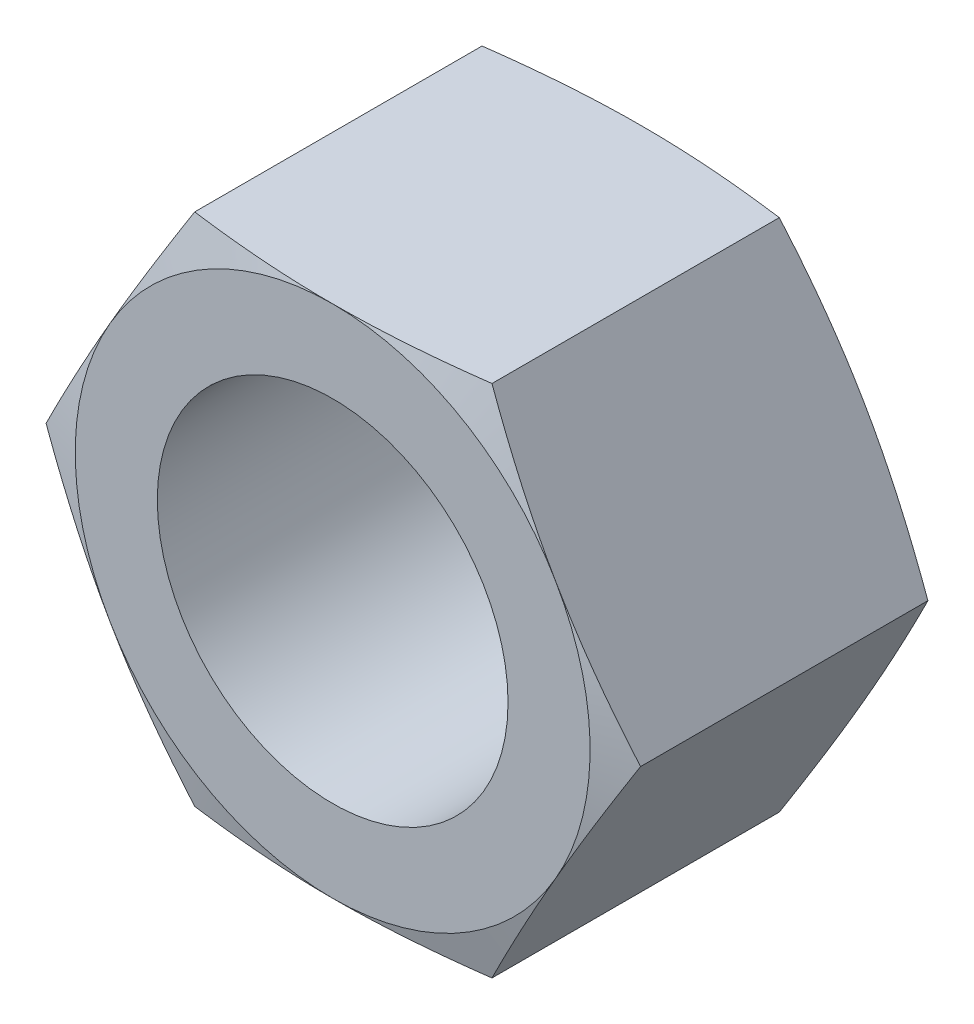
SolidWorks part; units mm, degrees
ref_plane "基准面1" through (0, 0, 0) normal (0, 0, 1) x (1, 0, 0)
ref_plane "基准面2" through (0, 0, 0) normal (0, 1, 0) x (1, 0, 0)
ref_plane "基准面3" through (0, 0, 0) normal (1, 0, 0) x (0, 0, -1)
sketch "尺寸草图" plane through (0, 0, 0) normal (0, 0, 1) x (1, 0, 0)
  line L0 (0, 0) -> (24.1005, 0)
  point P3 (30, 0)
  point P4 (1.5, 0)
  point P5 (50.85, 0)
  point P6 (26.4, 0)
  point P7 (6.4, 0)
  point P8 (46, 0)
sketch "草图1" plane through (0, 0, 0) normal (0, 0, 1) x (1, 0, 0)
  line L0 (-26.8088, 0) -> (37.1748, 0) construction
  line L1 (0, 25.0215) -> (0, -25.0215) construction
  line L3 (12.7125, 22.0187) -> (-12.7125, 22.0187)
  line L4 (-12.7125, 22.0187) -> (-25.425, 0)
  line L5 (-25.425, 0) -> (-12.7125, -22.0187)
  line L6 (-12.7125, -22.0187) -> (12.7125, -22.0187)
  line L7 (12.7125, -22.0187) -> (25.425, 0)
  line L8 (25.425, 0) -> (12.7125, 22.0187)
  circle A0 centre (0, 0) radius 22.0187 construction
  circle A1 centre (0, 0) radius 15
extrude "基体-拉伸" add sketch "草图1" along normal blind 26.4
cosmetic thread "装饰螺纹线1" parameters "D2"=31.5
sketch "草图2" plane through (0, 0, 0) normal (0, 0, -1) x (-1, 0, 0)
  line L0 (-12.7125, 22.0187) -> (12.7125, 22.0187) construction
  circle A0 centre (0, 0) radius 22.0187
  circle A1 centre (0, 0) radius 15 construction
extrude "切除-拉伸1" cut sketch "草图2" against normal blind 38 draft 75 flip side to cut
sketch "草图3" plane through (0, 0, 26.4) normal (0, 0, 1) x (1, 0, 0)
  line L0 (25.425, 0) -> (12.7125, 22.0187) construction
  circle A0 centre (0, 0) radius 22.0187
extrude "切除-拉伸2" cut sketch "草图3" against normal blind 38 draft 75 flip side to cut
chamfer "倒角1" [suppressed] distance 0.2 angle 45
equation "\"e@草图1\" = \"e@尺寸草图\""
equation "\"D@草图1\" = \"D@尺寸草图\""
equation "\"m@基体-拉伸\" = \"m@尺寸草图\""
equation "\"D2@装饰螺纹线1\" = 1.05 * \"D@尺寸草图\""
